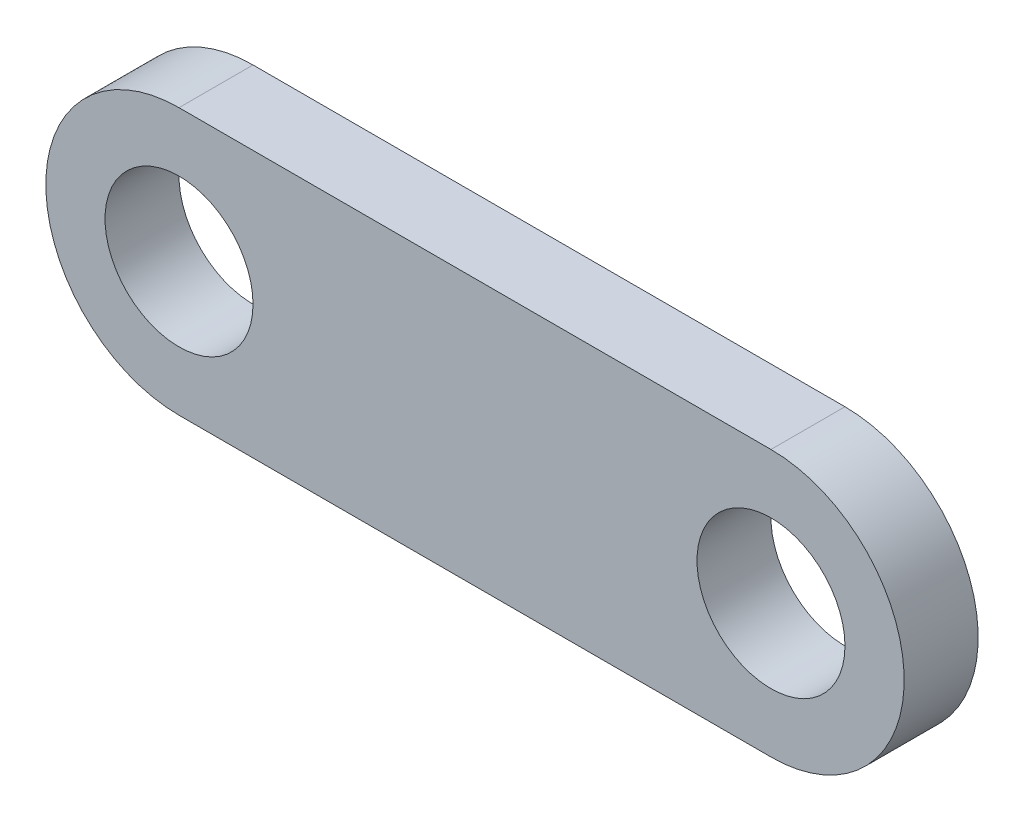
SolidWorks part; units mm, degrees
ref_plane "Plane1" through (0, 0, 0) normal (0, 0, 1) x (1, 0, 0)
ref_plane "Plane2" through (0, 0, 0) normal (0, 1, 0) x (1, 0, 0)
ref_plane "Plane3" through (0, 0, 0) normal (1, 0, 0) x (0, 0, -1)
sketch "Sketch1" plane through (0, 0, 0) normal (0, 0, 1) x (1, 0, 0)
  line L0 (0, 0) -> (40, 0) construction
  line L1 (0, 9) -> (40, 9)
  line L2 (0, -9) -> (40, -9)
  arc A0 (0, 9) -> (0, -9) centre (0, 0) ccw
  arc A1 (40, -9) -> (40, 9) centre (40, 0) ccw
  dimension "D1" = 9
  dimension "D2" = 9
  dimension "D4" = 40
extrude "Base-Extrude" add sketch "Sketch1" along normal blind 5
sketch "Sketch2" plane through (0, 0, 5) normal (0, 0, 1) x (1, 0, 0)
  circle A0 centre (0, 0) radius 5
  circle A1 centre (40, 0) radius 5
  dimension "D1" = 10
extrude "Cut-Extrude1" cut sketch "Sketch2" against normal through all
